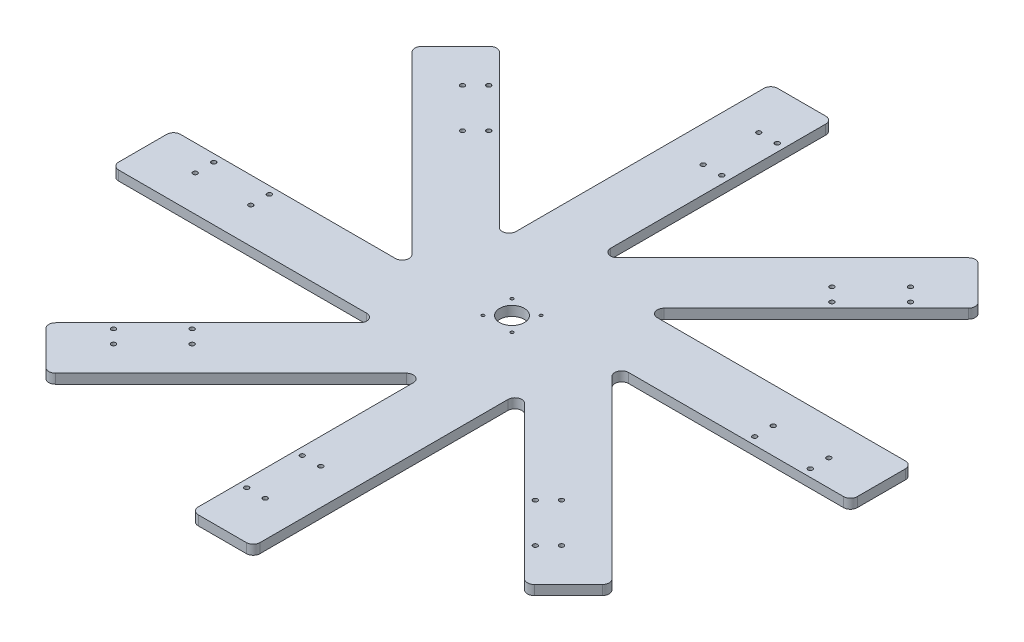
SolidWorks part; units mm, degrees
ref_plane "前视基准面" through (0, 0, 0) normal (0, 0, 1) x (1, 0, 0)
ref_plane "上视基准面" through (0, 0, 0) normal (0, 1, 0) x (1, 0, 0)
ref_plane "右视基准面" through (0, 0, 0) normal (1, 0, 0) x (0, 0, -1)
sketch "草图3" plane through (0, 0, 0) normal (0, 1, 0) x (1, 0, 0)
  circle A0 centre (0, 0) radius 50
  circle A1 centre (0, 0) radius 18
  dimension "D1" = 36
  dimension "D3" = 100
extrude "凸台-拉伸4" add sketch "草图3" along normal mid plane 14
sketch "草图4" plane through (0, 0, 0) normal (0, 1, 0) x (1, 0, 0)
  line L0 (0, 0) -> (0, 93.9744) construction
  line L1 (480, 13) -> (18, 13)
  line L2 (480, 13) -> (480, 103)
  line L3 (480, 103) -> (18, 103)
  line L4 (18, 13) -> (18, 103)
  line L5 (480, 13) -> (18, 103) construction
  line L6 (480, 103) -> (18, 13) construction
  line L7 (18, 13) -> (18, 0) construction
  line L8 (0, 0) -> (18, 0) construction
  circle A2 centre (0, 0) radius 18 construction
  point P0 (249, 58)
  dimension "D1" = 480
  dimension "D2" = 90
  dimension "D3" = 13
extrude "凸台-拉伸5" add sketch "草图4" along normal mid plane 14
sketch "草图5" plane through (0, 7, 0) normal (0, 1, 0) x (1, 0, 0)
  line L0 (480, 13) -> (480, 103) construction
  line L1 (329.5, 24) -> (410.5, 24) construction
  line L2 (329.5, 24) -> (329.5, 51) construction
  line L3 (329.5, 51) -> (410.5, 51) construction
  line L4 (410.5, 24) -> (410.5, 51) construction
  line L5 (329.5, 24) -> (410.5, 51) construction
  line L6 (329.5, 51) -> (410.5, 24) construction
  line L7 (48.2804, 13) -> (480, 13) construction
  line L8 (480, 103) -> (18, 103) construction
  circle A0 centre (329.5, 51) radius 3.3
  circle A1 centre (329.5, 24) radius 3.3
  circle A2 centre (410.5, 51) radius 3.3
  circle A3 centre (410.5, 24) radius 3.3
  point P0 (370, 37.5)
  dimension "D5" = 6.6
  dimension "D1" = 110
  dimension "D2" = 24.5
  dimension "D3" = 81
  dimension "D4" = 27
extrude "切除-拉伸7" cut sketch "草图5" against normal blind 30
fillet "圆角2" radius 10 2 edges at (480, 0, -103) (480, 0, -13)
pattern_circular "阵列(圆周)1" count 8 over 360 about axis through (0, 0, 0) along (0, 1, 0) of "凸台-拉伸5", "切除-拉伸7"
fillet "圆角1" radius 10 8 edges at (132.664, 0, -13) (103, 0, 84.6152) (13, 0, 132.664) (-84.6152, 0, 103) (-132.664, 0, 13) (-103, 0, -84.6152) (-13, 0, -132.664) (84.6152, 0, -103)
fillet "圆角3" radius 10 14 edges at (330.2189, 0, -348.6036) (266.5793, 0, -412.2433) (-13, 0, -480) (-103, 0, -480) (-412.2433, 0, -266.5793) (-348.6036, 0, -330.2189) (-480, 0, 13) (-480, 0, 103) (-330.2189, 0, 348.6036) (-266.5793, 0, 412.2433) (13, 0, 480) (103, 0, 480) (348.6036, 0, 330.2189) (412.2433, 0, 266.5793)
sketch "草图7" plane through (0, 7, 0) normal (0, 1, 0) x (1, 0, 0)
  circle A0 centre (0, 0) radius 30
  circle A1 centre (0, 0) radius 18
  circle A2 centre (0, 0) radius 18 construction
  dimension "D1" = 60
extrude "凸台-拉伸6" add sketch "草图7" along normal blind 15
sketch "草图8" plane through (0, 0, 0) normal (1, 0, 0) x (0, 0, -1)
  line L0 (0, 15) -> (0, 22) construction
  line L1 (18, 22) -> (-18, 22) construction
  circle A0 centre (0, 15) radius 2.75
  dimension "D1" = 5.5
  dimension "D2" = 7
extrude "切除-拉伸3" cut sketch "草图8" against normal blind 50
sketch "草图9" plane through (0, 0, 0) normal (1, 0, 0) x (0, 0, -1)
  circle A0 centre (0, 15) radius 5
  dimension "D1" = 10
extrude "切除-拉伸4" cut sketch "草图9" against normal blind 103 from offset 29 offset against normal yes
pattern_circular "阵列(圆周)2" count 4 over 360 about axis through (0, 0, 0) along (0, 1, 0) of "切除-拉伸4", "切除-拉伸3"
sketch "草图11" plane through (0, 7, 0) normal (0, 1, 0) x (1, 0, 0)
  circle A0 centre (0, 0) radius 87.3804
extrude "切除-拉伸5" cut sketch "草图11" along normal blind 51
sketch "草图12" plane through (0, 7, 0) normal (0, 1, 0) x (1, 0, 0)
  line L0 (0, 0) -> (21.2132, 21.2132) construction
  line L1 (0, 0) -> (11.073, 0) construction
  circle A0 centre (21.2132, 21.2132) radius 2.2
  dimension "D2" = 4.4
  dimension "D1" = 30
  dimension "D3" = 45
extrude "切除-拉伸6" cut sketch "草图12" against normal blind 51
pattern_circular "阵列(圆周)3" count 4 over 360 about axis through (0, 0, 0) along (0, 1, 0) of "切除-拉伸6"
